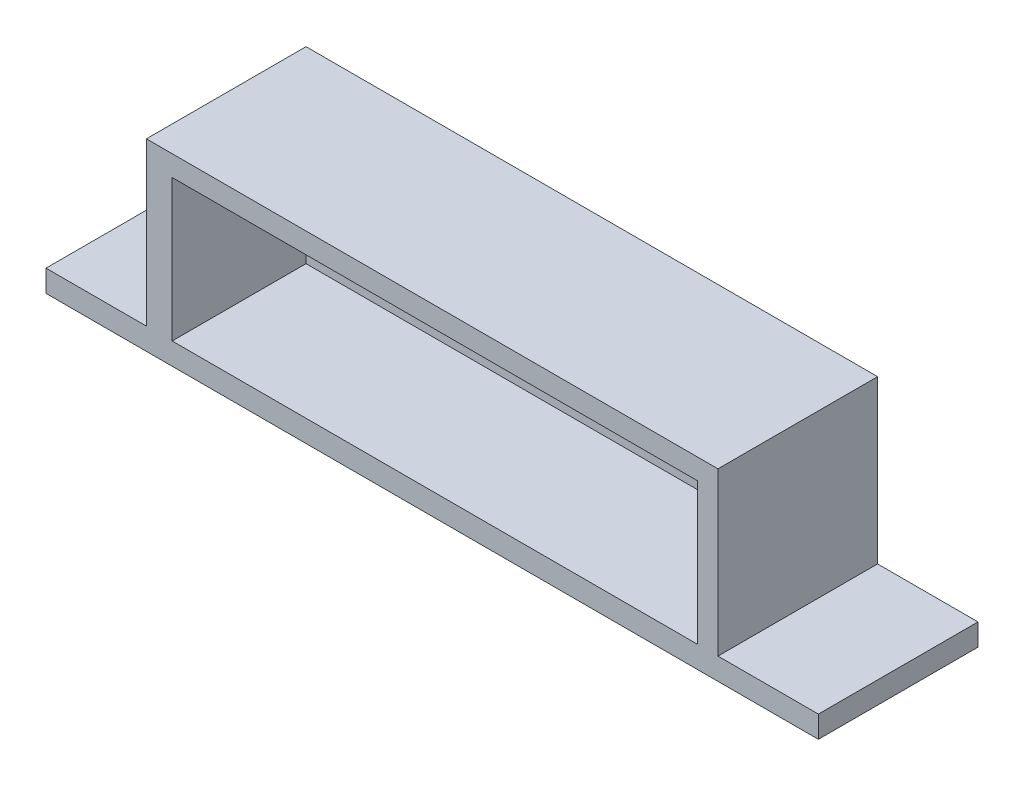
SolidWorks part; units mm, degrees
ref_plane "前视基准面" through (0, 0, 0) normal (0, 0, 1) x (1, 0, 0)
ref_plane "上视基准面" through (0, 0, 0) normal (0, 1, 0) x (1, 0, 0)
ref_plane "右视基准面" through (0, 0, 0) normal (1, 0, 0) x (0, 0, -1)
sketch "草图1" plane through (0, 0, 0) normal (0, 1, 0) x (1, 0, 0)
  line L1 (-150, -31) -> (150, -31)
  line L2 (-150, -31) -> (-150, 31)
  line L3 (-150, 31) -> (150, 31)
  line L4 (150, -31) -> (150, 31)
  line L5 (-150, -31) -> (150, 31) construction
  line L6 (-150, 31) -> (150, -31) construction
  point P0 (0, 0)
  dimension "D1" = 62
  dimension "D2" = 300
extrude "凸台-拉伸1" add sketch "草图1" along normal mid plane 10
sketch "草图2" plane through (0, -5, 0) normal (0, -1, 0) x (1, 0, 0)
  line L0 (150, 31) -> (150, -31) construction
  line L1 (-148.1209, 19) -> (150, 19)
  line L2 (-148.1209, 19) -> (-148.1209, 31)
  line L3 (-148.1209, 31) -> (150, 31)
  line L4 (150, 19) -> (150, 31)
  line L5 (-150, 31) -> (150, 31) construction
  point P7 (0, 0)
  point P8 (0, 0)
  point P9 (-148.1209, 31)
  dimension "D1" = 12
extrude "切除-拉伸1" cut sketch "草图2" against normal blind 1.5
sketch "草图3" plane through (0, -5, 0) normal (0, -1, 0) x (1, 0, 0)
  line L1 (-150, 31) -> (-135, 31)
  line L2 (-150, 31) -> (-150, -31)
  line L3 (-150, -31) -> (-135, -31)
  line L4 (-135, 31) -> (-135, -31)
  line L5 (-150, -31) -> (150, -31) construction
  line L6 (150, 31) -> (136, 31)
  line L7 (150, 31) -> (150, -31)
  line L8 (150, -31) -> (136, -31)
  line L9 (136, 31) -> (136, -31)
  line L10 (150, 19) -> (150, -31) construction
  line L11 (150, 31) -> (-148.1209, 31) construction
  point P5 (136, -32.2893)
  point P12 (0, 0)
  point P13 (0, 0)
  point P14 (0, 0)
  point P16 (-135, -37.5986)
  point P17 (0, 0)
  point P18 (0, 0)
  point P19 (0, 0)
  point P20 (0, 0)
  point P21 (150, -31)
  point P24 (136, 35.4167)
  dimension "D1" = 15
  dimension "D2" = 14
extrude "切除-拉伸2" cut sketch "草图3" against normal blind 1.5
sketch "草图4" plane through (0, 5, 0) normal (0, 1, 0) x (1, 0, 0)
  line L0 (-111, -31) -> (-111, 31)
  line L1 (-111, 31) -> (111, 31)
  line L2 (111, 31) -> (111, -31)
  line L3 (111, -31) -> (103, -31)
  line L4 (-150, -31) -> (150, -31) construction
  line L5 (103, -31) -> (103, 21)
  line L6 (103, 21) -> (-101, 21)
  line L7 (-101, 21) -> (-101, -31)
  line L8 (-101, -31) -> (-111, -31)
  line L9 (150, 31) -> (-150, 31) construction
  line L10 (150, -31) -> (150, 31) construction
  line L11 (-150, 31) -> (-150, -31) construction
  point P5 (0, 0)
  point P8 (0, 0)
  point P13 (0, 0)
  point P15 (-116.8413, -31)
extrude "凸台-拉伸2" add sketch "草图4" along normal blind 55
sketch "草图5" plane through (0, 60, 0) normal (0, 1, 0) x (1, 0, 0)
  line L1 (-111, -31) -> (111, -31)
  line L2 (-111, -31) -> (-111, 31)
  line L3 (-111, 31) -> (111, 31)
  line L4 (111, -31) -> (111, 31)
  point P5 (0, 0)
  point P6 (-123, -31)
extrude "凸台-拉伸3" add sketch "草图5" along normal blind 8
sketch "草图6" plane through (0, 0, -21) normal (0, 0, 1) x (1, 0, 0)
  line L0 (-101, 5) -> (103, 5) construction
  line L1 (-81, 19) -> (-39.6667, 19)
  line L2 (-81, 19) -> (-81, 46)
  line L3 (-81, 46) -> (-39.6667, 46)
  line L4 (-39.6667, 19) -> (-39.6667, 46)
  line L5 (-81, 19) -> (-39.6667, 46) construction
  line L6 (-81, 46) -> (-39.6667, 19) construction
  line L7 (41.6667, 19) -> (83, 19)
  line L8 (41.6667, 19) -> (41.6667, 46)
  line L9 (41.6667, 46) -> (83, 46)
  line L10 (83, 19) -> (83, 46)
  line L11 (41.6667, 19) -> (83, 46) construction
  line L12 (41.6667, 46) -> (83, 19) construction
  line L13 (-19.6667, 19) -> (21.6667, 19)
  line L14 (-19.6667, 19) -> (-19.6667, 46)
  line L15 (-19.6667, 46) -> (21.6667, 46)
  line L16 (21.6667, 19) -> (21.6667, 46)
  line L17 (-19.6667, 19) -> (21.6667, 46) construction
  line L18 (-19.6667, 46) -> (21.6667, 19) construction
  line L19 (-101, 60) -> (103, 60) construction
  line L20 (103, 60) -> (103, 5) construction
  line L21 (-101, 60) -> (-101, 5) construction
  point P0 (-60.3333, 32.5)
  point P5 (62.3333, 32.5)
  point P10 (0, 33.1532)
  dimension "D1" = 14
  dimension "D2" = 14
  dimension "D3" = 20
  dimension "D4" = 20
  dimension "D5" = 20
  dimension "D6" = 20
extrude "切除-拉伸3" cut sketch "草图6" against normal up to next
fillet "圆角1" radius 5 12 edges at (-19.6667, 19, -26) (-19.6667, 46, -26) (21.6667, 46, -26) (41.6667, 19, -26) (41.6667, 46, -26) (83, 46, -26) (83, 19, -26) (-81, 19, -26) (-81, 46, -26) (-39.6667, 46, -26) (-39.6667, 19, -26) (21.6667, 19, -26)
sketch "草图7" plane through (0, 0, 0) normal (0, 0, 1) x (1, 0, 0)
  line L0 (111, 40) -> (121, 40)
  line L1 (111, 68) -> (111, 5) construction
  line L2 (121, 40) -> (146, 15)
  line L3 (146, 15) -> (146, 5)
  line L4 (146, 5) -> (116, 5)
  line L5 (111, 5) -> (150, 5) construction
  line L6 (116, 5) -> (111, 10)
  line L7 (111, 10) -> (111, 40)
  line L9 (150, 5) -> (150, -3.5) construction
  dimension "D1" = 5
  dimension "D2" = 5
  dimension "D3" = 10
  dimension "D4" = 10
  dimension "D5" = 4
extrude "凸台-拉伸4" [suppressed] add sketch "草图7" along normal mid plane 8
equation "\"D5@草图4\"=\"D4@草图4\""
